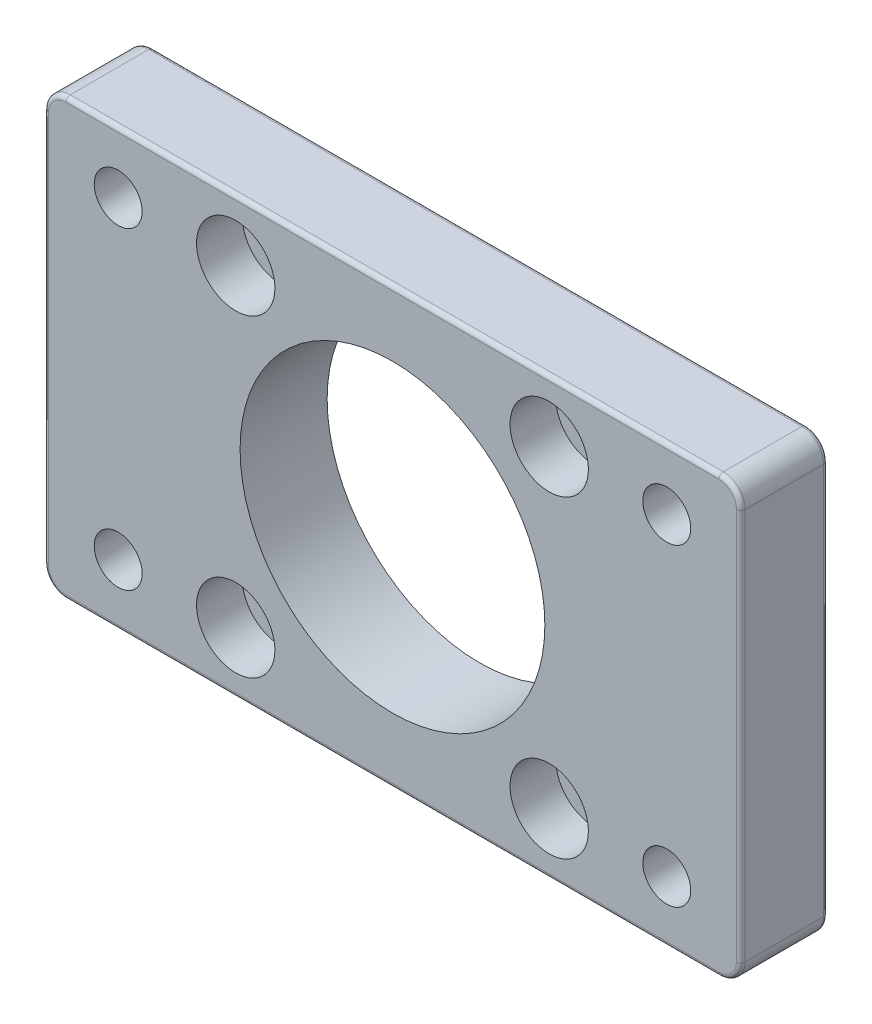
SolidWorks part; units mm, degrees
ref_plane "Front Plane" through (0, 0, 0) normal (0, 0, 1) x (1, 0, 0)
ref_plane "Top Plane" through (0, 0, 0) normal (0, 1, 0) x (1, 0, 0)
ref_plane "Right Plane" through (0, 0, 0) normal (1, 0, 0) x (0, 0, -1)
sketch "Sketch1" plane through (0, 0, 0) normal (0, 0, 1) x (1, 0, 0)
  line L1 (80, -50) -> (-80, -50)
  line L2 (80, -50) -> (80, 50)
  line L3 (80, 50) -> (-80, 50)
  line L4 (-80, -50) -> (-80, 50)
  line L5 (80, -50) -> (-80, 50) construction
  line L6 (80, 50) -> (-80, -50) construction
  circle A0 centre (0, 0) radius 35
  point P0 (0, 0)
  dimension "D3" = 70
  dimension "D1" = 160
  dimension "D2" = 100
extrude "Boss-Extrude1" add sketch "Sketch1" along normal blind 20
fillet "Fillet1" radius 5 4 edges at (80, -50, 10) (-80, -50, 10) (-80, 50, 10) (80, 50, 10)
hole_wizard "Hole Spec (per socket head cap screw type) 1" positions "Sketch3" profile "Sketch4" counterbore size "M10" standard "GB" end condition through all
sketch "Sketch3" plane through (0, 0, 20) normal (0, 0, 1) x (1, 0, 0)
  line L0 (0, 0) -> (0, 65.5217) construction
  line L2 (0, 0) -> (-60.9306, 0) construction
  point P0 (-36, 36)
  point P2 (36, 36)
  point P4 (-36, -36)
  point P6 (36, -36)
  dimension "D1" = 72
  dimension "D2" = 72
sketch "Sketch4" plane through (-36, 36, 20) normal (1, 0, 0) x (0, -1, 0)
  line L0 (0, 0) -> (0, 20)
  line L1 (0, 20) -> (5.5, 20)
  line L3 (5.5, 20) -> (5.5, 10.5)
  line L4 (5.5, 10.5) -> (9, 10.5)
  line L5 (9, 10.5) -> (9, 0)
  line L7 (9, 0) -> (0, 0)
  line L11 (0, -6.35) -> (0, 107.95) construction
  dimension "通孔孔直径" = 11
  dimension "通孔孔深度" = 20
  dimension "柱形沉头孔直径" = 18
  dimension "柱形沉头孔深度" = 10.5
hole_wizard "Hole Spec (per socket head cap screw type) 2" positions "Sketch5" profile "Sketch6" counterbore size "M10" standard "GB" end condition through all
sketch "Sketch5" plane through (0, 0, 0) normal (0, 0, -1) x (-1, 0, 0)
  line L0 (0, 0) -> (0, 69.5089) construction
  line L2 (0, 0) -> (-93.9305, 0) construction
  point P0 (-63, 36)
  point P2 (63, 36)
  point P4 (-63, -36)
  point P6 (63, -36)
  dimension "D1" = 126
  dimension "D2" = 72
sketch "Sketch6" plane through (63, 36, 0) normal (1, 0, 0) x (0, 1, 0)
  line L0 (0, 0) -> (0, 20)
  line L1 (0, 20) -> (5.5, 20)
  line L3 (5.5, 20) -> (5.5, 11)
  line L4 (5.5, 11) -> (9, 11)
  line L5 (9, 11) -> (9, 0)
  line L7 (9, 0) -> (0, 0)
  line L11 (0, -6.35) -> (0, 107.95) construction
  dimension "通孔孔直径" = 11
  dimension "通孔孔深度" = 20
  dimension "柱形沉头孔直径" = 18
  dimension "柱形沉头孔深度" = 11
fillet "Fillet2" radius 1 16 edges at (78.5355, 48.5355, 20) (80, 0, 20) (78.5355, -48.5355, 20) (0, -50, 20) (-78.5355, -48.5355, 20) (-80, 0, 20) (-78.5355, 48.5355, 20) (78.5355, 48.5355, 0) (80, 0, 0) (78.5355, -48.5355, 0) (0, -50, 0) (-78.5355, -48.5355, 0) (-80, 0, 0) (-78.5355, 48.5355, 0) (0, 50, 20) (0, 50, 0)
